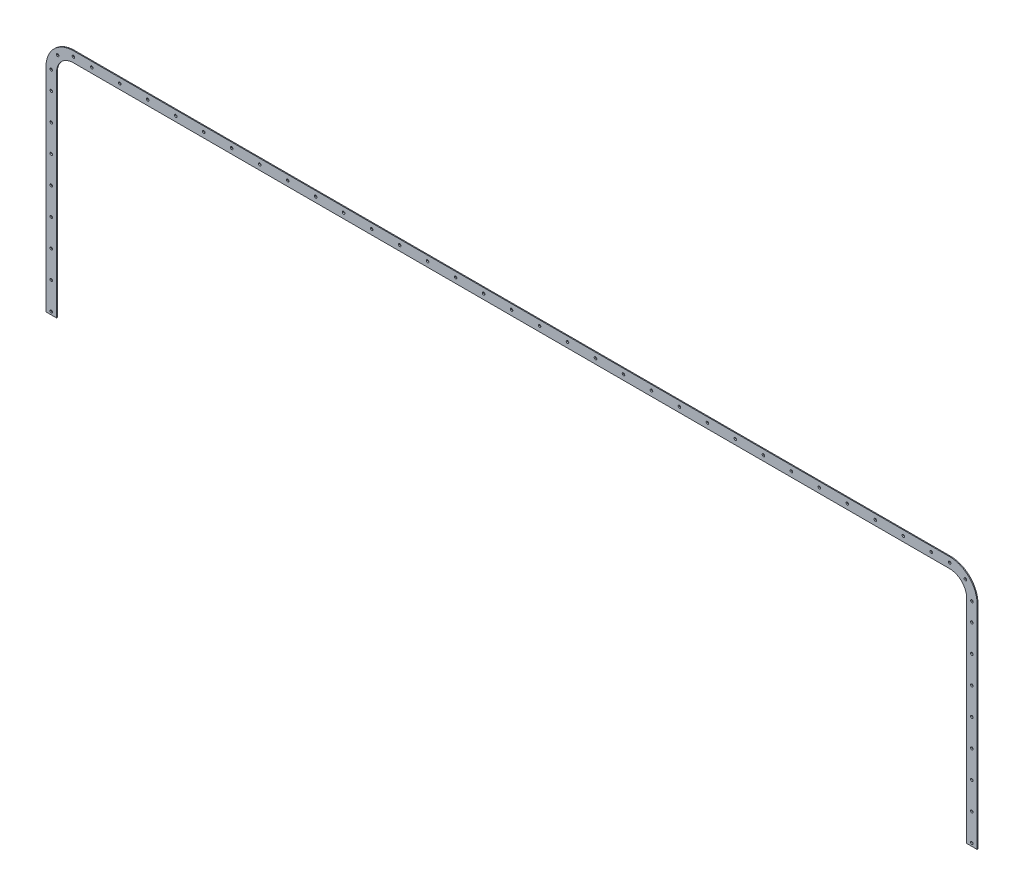
SolidWorks part; units mm, degrees
ref_plane "Front Plane" through (0, 0, 0) normal (0, 0, 1) x (1, 0, 0)
ref_plane "Top Plane" through (0, 0, 0) normal (0, 1, 0) x (1, 0, 0)
ref_plane "Right Plane" through (0, 0, 0) normal (1, 0, 0) x (0, 0, -1)
sketch "Sketch2" plane through (0, 0, 0) normal (0, 0, 1) x (1, 0, 0)
  line L0 (0, 0) -> (0, 712)
  line L1 (92, 804) -> (3029, 804)
  line L2 (3121, 712) -> (3121, 0)
  line L3 (35, 0) -> (35, 712)
  line L4 (92, 769) -> (3029, 769)
  line L5 (3086, 712) -> (3086, 0)
  line L6 (35, 0) -> (0, 0)
  line L7 (3086, 0) -> (3121, 0)
  arc A0 (3121, 712) -> (3029, 804) centre (3029, 712) ccw
  arc A1 (0, 712) -> (92, 804) centre (92, 712) cw
  arc A2 (35, 712) -> (92, 769) centre (92, 712) cw
  arc A3 (3086, 712) -> (3029, 769) centre (3029, 712) ccw
  point P8 (3121, 804)
  point P11 (0, 804)
  dimension "D3" = 92
  dimension "D1" = 3121
  dimension "D2" = 804
  dimension "D4" = 35
extrude "Boss-Extrude1" add sketch "Sketch2" along normal blind 3.2
sketch "Sketch3" plane through (0, 0, 3.2) normal (0, 0, 1) x (1, 0, 0)
  line L0 (0, 0) -> (35, 0) construction
  line L11 (1560.5, 786.5) -> (1560.5, 1049.1644) construction
  line L12 (39.3205, 764.6795) -> (92, 712) construction
  line L13 (3103.5, 712) -> (3103.5, 0)
  line L14 (92, 786.5) -> (3029, 786.5)
  line L15 (17.5, 0) -> (17.5, 712)
  line L16 (3103.5, 712) -> (3103.5, 0) construction
  line L17 (92, 786.5) -> (3029, 786.5) construction
  line L18 (17.5, 0) -> (17.5, 712) construction
  line L19 (3081.6795, 764.6795) -> (3029, 712) construction
  circle A0 centre (17.5, 10) radius 4.3
  circle A1 centre (92, 786.5) radius 4.3
  circle A2 centre (17.5, 712) radius 4.3
  circle A3 centre (3029, 786.5) radius 4.3
  circle A4 centre (3103.5, 712) radius 4.3
  circle A7 centre (17.5, 101.5) radius 4.3
  circle A8 centre (17.5, 193) radius 4.3
  arc A9 (3103.5, 712) -> (3029, 786.5) centre (3029, 712) ccw
  arc A10 (92, 786.5) -> (17.5, 712) centre (92, 712) ccw
  arc A11 (3103.5, 712) -> (3029, 786.5) centre (3029, 712) ccw construction
  arc A12 (92, 786.5) -> (17.5, 712) centre (92, 712) ccw construction
  circle A13 centre (17.5, 284.5) radius 4.3
  circle A14 centre (17.5, 376) radius 4.3
  circle A15 centre (17.5, 467.5) radius 4.3
  circle A16 centre (17.5, 559) radius 4.3
  circle A17 centre (17.5, 650.5) radius 4.3
  circle A18 centre (3103.5, 650.5) radius 4.3
  circle A19 centre (3103.5, 559) radius 4.3
  circle A20 centre (3103.5, 467.5) radius 4.3
  circle A21 centre (3103.5, 376) radius 4.3
  circle A22 centre (3103.5, 284.5) radius 4.3
  circle A23 centre (3103.5, 193) radius 4.3
  circle A24 centre (3103.5, 101.5) radius 4.3
  circle A25 centre (3103.5, 10) radius 4.3
  circle A26 centre (39.3205, 764.6795) radius 4.3
  circle A30 centre (3081.6795, 764.6795) radius 4.3
  circle A32 centre (153.5, 786.5) radius 4.3
  circle A33 centre (2967.5, 786.5) radius 4.3
  circle A34 centre (247.3, 786.5) radius 4.3
  circle A35 centre (341.1, 786.5) radius 4.3
  circle A36 centre (434.9, 786.5) radius 4.3
  circle A37 centre (528.7, 786.5) radius 4.3
  circle A38 centre (622.5, 786.5) radius 4.3
  circle A39 centre (716.3, 786.5) radius 4.3
  circle A40 centre (810.1, 786.5) radius 4.3
  circle A41 centre (903.9, 786.5) radius 4.3
  circle A42 centre (997.7, 786.5) radius 4.3
  circle A43 centre (1091.5, 786.5) radius 4.3
  circle A44 centre (1185.3, 786.5) radius 4.3
  circle A45 centre (1279.1, 786.5) radius 4.3
  circle A46 centre (1372.9, 786.5) radius 4.3
  circle A47 centre (1466.7, 786.5) radius 4.3
  circle A48 centre (1560.5, 786.5) radius 4.3
  circle A49 centre (1654.3, 786.5) radius 4.3
  circle A50 centre (1748.1, 786.5) radius 4.3
  circle A51 centre (1841.9, 786.5) radius 4.3
  circle A52 centre (1935.7, 786.5) radius 4.3
  circle A53 centre (2029.5, 786.5) radius 4.3
  circle A54 centre (2123.3, 786.5) radius 4.3
  circle A55 centre (2217.1, 786.5) radius 4.3
  circle A56 centre (2310.9, 786.5) radius 4.3
  circle A57 centre (2404.7, 786.5) radius 4.3
  circle A58 centre (2498.5, 786.5) radius 4.3
  circle A59 centre (2592.3, 786.5) radius 4.3
  circle A60 centre (2686.1, 786.5) radius 4.3
  circle A61 centre (2779.9, 786.5) radius 4.3
  circle A62 centre (2873.7, 786.5) radius 4.3
  point P5 (17.5, 0)
  dimension "D1" = 8.6
  dimension "D5" = 8.6
  dimension "D6" = 8.6
  dimension "D2" = 10
  dimension "D7" = 30
  dimension "D3" = 17.5
  dimension "D4" = 8
extrude "Cut-Extrude1" cut sketch "Sketch3" against normal blind 2.05 draft 45
sketch "Sketch4" plane through (0, 0, 1.15) normal (0, 0, 1) x (1, 0, 0)
  circle A0 centre (17.5, 101.5) radius 2.25 construction
  circle A1 centre (17.5, 10) radius 2.25 construction
  circle A2 centre (17.5, 101.5) radius 2.25
  circle A3 centre (17.5, 10) radius 2.25
  circle A4 centre (341.1, 786.5) radius 2.25 construction
  circle A5 centre (247.3, 786.5) radius 2.25 construction
  circle A6 centre (153.5, 786.5) radius 2.25 construction
  circle A7 centre (39.3205, 764.6795) radius 2.25 construction
  circle A8 centre (17.5, 650.5) radius 2.25 construction
  circle A9 centre (17.5, 559) radius 2.25 construction
  circle A10 centre (17.5, 467.5) radius 2.25 construction
  circle A11 centre (17.5, 376) radius 2.25 construction
  circle A12 centre (17.5, 284.5) radius 2.25 construction
  circle A13 centre (17.5, 193) radius 2.25 construction
  circle A14 centre (341.1, 786.5) radius 2.25
  circle A15 centre (247.3, 786.5) radius 2.25
  circle A16 centre (153.5, 786.5) radius 2.25
  circle A17 centre (39.3205, 764.6795) radius 2.25
  circle A18 centre (17.5, 650.5) radius 2.25
  circle A19 centre (17.5, 559) radius 2.25
  circle A20 centre (17.5, 467.5) radius 2.25
  circle A21 centre (17.5, 376) radius 2.25
  circle A22 centre (17.5, 284.5) radius 2.25
  circle A23 centre (17.5, 193) radius 2.25
  circle A24 centre (528.7, 786.5) radius 2.25
  circle A25 centre (434.9, 786.5) radius 2.25
  circle A26 centre (434.9, 786.5) radius 2.25
  circle A27 centre (622.5, 786.5) radius 2.25
  circle A28 centre (716.3, 786.5) radius 2.25
  circle A29 centre (810.1, 786.5) radius 2.25
  circle A30 centre (903.9, 786.5) radius 2.25
  circle A31 centre (997.7, 786.5) radius 2.25
  circle A32 centre (1091.5, 786.5) radius 2.25
  circle A33 centre (1185.3, 786.5) radius 2.25
  circle A34 centre (1279.1, 786.5) radius 2.25
  circle A35 centre (1372.9, 786.5) radius 2.25
  circle A36 centre (1466.7, 786.5) radius 2.25
  circle A37 centre (1560.5, 786.5) radius 2.25
  circle A38 centre (1654.3, 786.5) radius 2.25
  circle A39 centre (1748.1, 786.5) radius 2.25
  circle A40 centre (1841.9, 786.5) radius 2.25
  circle A41 centre (1935.7, 786.5) radius 2.25
  circle A42 centre (2029.5, 786.5) radius 2.25
  circle A43 centre (2123.3, 786.5) radius 2.25
  circle A44 centre (2217.1, 786.5) radius 2.25
  circle A45 centre (2310.9, 786.5) radius 2.25
  circle A46 centre (2404.7, 786.5) radius 2.25
  circle A47 centre (2498.5, 786.5) radius 2.25
  circle A48 centre (2592.3, 786.5) radius 2.25
  circle A49 centre (2686.1, 786.5) radius 2.25
  circle A50 centre (2779.9, 786.5) radius 2.25
  circle A51 centre (2873.7, 786.5) radius 2.25
  circle A52 centre (2967.5, 786.5) radius 2.25
  circle A53 centre (3103.5, 559) radius 2.25
  circle A54 centre (3081.6795, 764.6795) radius 2.25
  circle A55 centre (3081.6795, 764.6795) radius 2.25
  circle A56 centre (3103.5, 650.5) radius 2.25
  circle A57 centre (3103.5, 650.5) radius 2.25
  circle A58 centre (3103.5, 467.5) radius 2.25
  circle A59 centre (3103.5, 376) radius 2.25
  circle A60 centre (3103.5, 284.5) radius 2.25
  circle A61 centre (3103.5, 193) radius 2.25
  circle A62 centre (3103.5, 101.5) radius 2.25
  circle A63 centre (3103.5, 10) radius 2.25
  circle A65 centre (17.5, 712) radius 2.25
  circle A66 centre (17.5, 712) radius 2.25
  circle A67 centre (92, 786.5) radius 2.25
  circle A68 centre (92, 786.5) radius 2.25
  circle A69 centre (3029, 786.5) radius 2.25
  circle A70 centre (3029, 786.5) radius 2.25
  circle A71 centre (3103.5, 712) radius 2.25
  circle A72 centre (3103.5, 712) radius 2.25
  dimension "D1" = 0
  dimension "D3" = 0
  dimension "D4" = 0
  dimension "D6" = 0
  dimension "D7" = 0
  dimension "D8" = 0
  dimension "D9" = 0
  dimension "D2" = 28
  dimension "D5" = 8
extrude "Cut-Extrude2" cut sketch "Sketch4" against normal blind 2.05
sketch "Sketch5" plane through (0, 0, 0) normal (0, 0, -1) x (-1, 0, 0)
  line L8 (-35, 0) -> (0, 0)
  line L9 (0, 0) -> (0, 712)
  line L10 (-92, 804) -> (-3029, 804)
  line L11 (-3121, 712) -> (-3121, 0)
  line L12 (-3121, 0) -> (-3086, 0)
  line L13 (-3086, 0) -> (-3086, 712)
  line L14 (-3029, 769) -> (-92, 769)
  line L15 (-35, 712) -> (-35, 0)
  line L16 (-35, 0) -> (0, 0)
  line L17 (0, 0) -> (0, 712)
  line L18 (-92, 804) -> (-3029, 804)
  line L19 (-3121, 712) -> (-3121, 0)
  line L20 (-3121, 0) -> (-3086, 0)
  line L21 (-3086, 0) -> (-3086, 712)
  line L22 (-3029, 769) -> (-92, 769)
  line L23 (-35, 712) -> (-35, 0)
  arc A4 (0, 712) -> (-92, 804) centre (-92, 712) ccw
  arc A5 (-3029, 804) -> (-3121, 712) centre (-3029, 712) ccw
  arc A6 (-3029, 769) -> (-3086, 712) centre (-3029, 712) ccw
  arc A7 (-35, 712) -> (-92, 769) centre (-92, 712) ccw
  arc A8 (0, 712) -> (-92, 804) centre (-92, 712) ccw
  arc A9 (-3029, 804) -> (-3121, 712) centre (-3029, 712) ccw
  arc A10 (-3029, 769) -> (-3086, 712) centre (-3029, 712) ccw
  arc A11 (-35, 712) -> (-92, 769) centre (-92, 712) ccw
  dimension "D1" = 0
extrude "Cut-Extrude3" cut sketch "Sketch5" against normal blind 0.2
